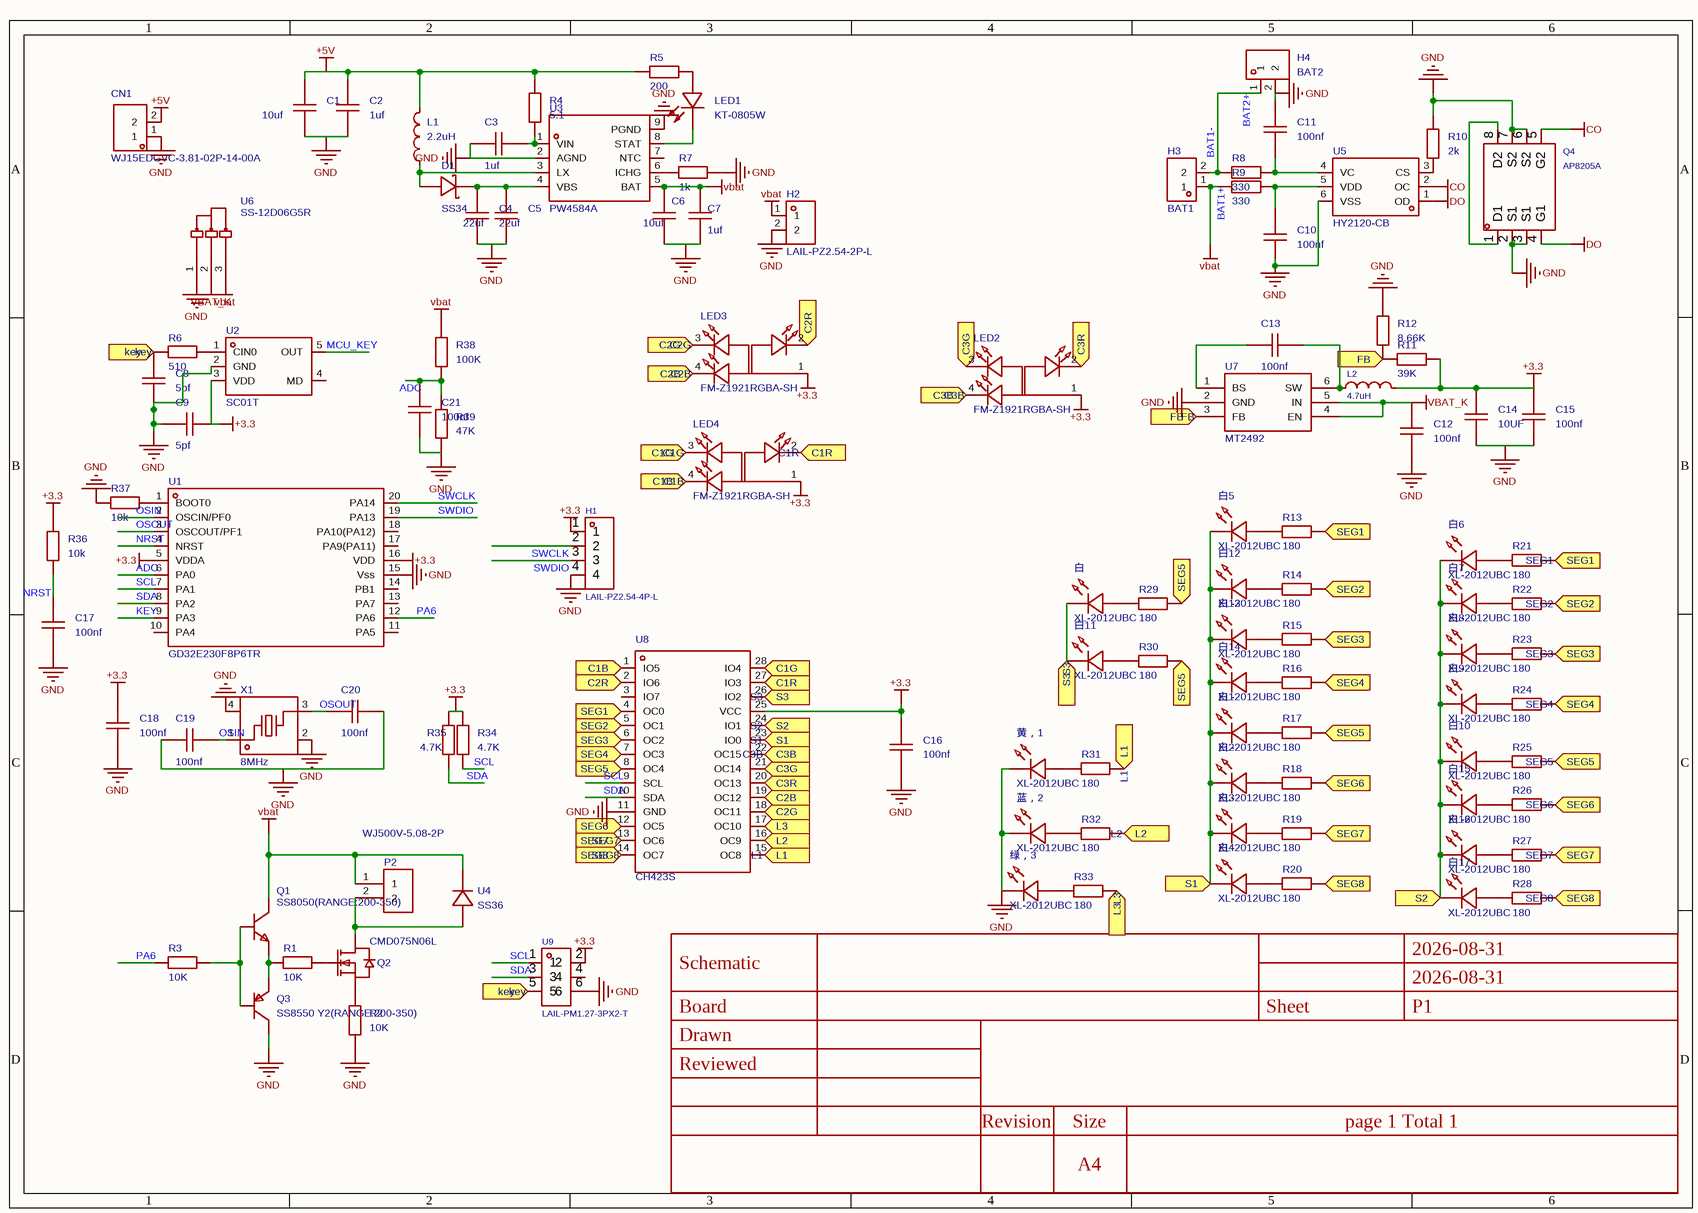
[diagram p0: MISC80546-2.schdoc]
# Altium schematic sheet MISC80546-2.schdoc
size 297 x 209 mm; Version: V1.0; @Project Name: MISC80546; @Update Date: 2026-08-31; @Create Date: 2026-08-31; @Board Name: MISC80546; @Create Time: 14:55:22; @Page Count: 1; @Page No: 1; @Schematic Name: MISC80546; @Update Time: 14:55:22; Size: A4

## Parts
C1  10uf  [C0603]
C2  1uf  [C0603]
C3  1uf  [C0603]
C4  22uf  [C0603]
C5  22uf  [C0603]
C6  10uf  [C0603]
C7  1uf  [C0603]
C8  5pf  [C0603]
C9  5pf  [C0603]
C10  100nf  [C0603]
C11  100nf  [C0603]
C12  100nf  [C0603]
C13  100nf  [C0603]
C14  10UF  [C0603]
C15  100nf  [C0603]
C16  100nf  [C0603]
C17  100nf  [C0603]
C18  100nf  [C0603]
C19  100nf  [C0603]
C20  100nf  [C0603]
C21  100nf  [C0603]
CN1  WJ15EDGVC-3.81-02P-14-00A  [CONN-TH_WJ15EDGVC-3.81-2P]
D1  SS34  [SMA_L4.3-W2.6-LS5.2-RD]
H1  LAIL-PZ2.54-4P-L  [CONN-TH_LAIL-PZ2.54-4P-L]
H2  LAIL-PZ2.54-2P-L  [CONN-TH_LAIL-PZ2.54-2P-L]
H3  BAT1  [CONN-TH_LAIL-PZ2.54-2P-L]
H4  BAT2  [CONN-TH_LAIL-PZ2.54-2P-L]
L1  2.2uH  [IND-SMD_L4.0-W4.0_LQH44PN2R2MP0L]
L2  4.7uH  [IND-SMD_L4.0-W4.0_SMNR4012]
LED1  KT-0805W  [LED0805-R-RD]
LED2  FM-Z1921RGBA-SH  [LED-ARRAY-SMD_4P-L2.2-W2.1-BR]
LED3  FM-Z1921RGBA-SH  [LED-ARRAY-SMD_4P-L2.2-W2.1-BR]
LED4  FM-Z1921RGBA-SH  [LED-ARRAY-SMD_4P-L2.2-W2.1-BR]
P2  WJ500V-5.08-2P  [CONN-TH_2P-P5.00_WJ500V-5.08-2P]
Q1  SS8050(RANGE:200-350)  [SOT-23-3_L2.9-W1.3-P1.90-LS2.4-BR]
Q2  CMD075N06L  [TO-252-2_L6.6-W6.1-P4.57-LS9.9-BR-CW]
Q3  SS8550 Y2(RANGE:200-350)  [SOT-23-3_L2.9-W1.3-P1.90-LS2.4-BR]
Q4  AP8205A  [TSSOP-8_L4.4-W3.0-P0.65-LS6.4-BL-2]
R1  10K  [R0603]
R2  10K  [R0603]
R3  10K  [R0603]
R4  5.1  [R0603]
R5  200  [R0603]
R6  510  [R0603]
R7  1k  [R0603]
R8  330  [R0603]
R9  330  [R0603]
R10  2k  [R0603]
R11  39K  [R0603]
R12  8.66K  [R0603]
R13  180  [R0603]
R14  180  [R0603]
R15  180  [R0603]
R16  180  [R0603]
R17  180  [R0603]
R18  180  [R0603]
R19  180  [R0603]
R20  180  [R0603]
R21  180  [R0603]
R22  180  [R0603]
R23  180  [R0603]
R24  180  [R0603]
R25  180  [R0603]
R26  180  [R0603]
R27  180  [R0603]
R28  180  [R0603]
R29  180  [R0603]
R30  180  [R0603]
R31  180  [R0603]
R32  180  [R0603]
R33  180  [R0603]
R34  4.7K  [R0603]
R35  4.7K  [R0603]
R36  10k  [R0603]
R37  10k  [R0603]
R38  100K  [R0603]
R39  47K  [R0603]
U1  GD32E230F8P6TR  [TSSOP-20_L6.5-W4.4-P0.65-LS6.4-BL]
U2  SC01T  [SOT-23-5_L2.9-W1.6-P0.95-LS2.8-BR]
U3  PW4584A  [ESOP-8_L4.9-W3.9-P1.27-LS6.0-BL-EP-1]
U4  SS36  [SMA_L4.3-W2.6-LS5.1-RD]
U5  HY2120-CB  [SOT-23-6_L2.9-W1.6-P0.95-LS2.8-BR]
U6  SS-12D06G5R  [SW-TH_SS-12D06G5R]
U7  MT2492  [SOT-23-6_L2.9-W1.6-P0.95-LS2.8-BL_3]
U8  CH423S  [SOP-28_L17.9-W7.5-P1.27-LS10.3-BL]
U9  LAIL-PM1.27-3PX2-T  [HDR-SMD_6P-P1.27_LAIL-PM1.27-3PX2-T]
X1  8MHz  [CRYSTAL-SMD_4P-L3.2-W2.5-BL]
白  XL-2012UBC  [LED0805-RD]
白1  XL-2012UBC  [LED0805-RD]
白2  XL-2012UBC  [LED0805-RD]
白3  XL-2012UBC  [LED0805-RD]
白4  XL-2012UBC  [LED0805-RD]
白5  XL-2012UBC  [LED0805-RD]
白6  XL-2012UBC  [LED0805-RD]
白7  XL-2012UBC  [LED0805-RD]
白8  XL-2012UBC  [LED0805-RD]
白9  XL-2012UBC  [LED0805-RD]
白10  XL-2012UBC  [LED0805-RD]
白11  XL-2012UBC  [LED0805-RD]
白12  XL-2012UBC  [LED0805-RD]
白13  XL-2012UBC  [LED0805-RD]
白14  XL-2012UBC  [LED0805-RD]
白15  XL-2012UBC  [LED0805-RD]
白16  XL-2012UBC  [LED0805-RD]
白17  XL-2012UBC  [LED0805-RD]
绿，3  XL-2012UBC  [LED0805-RD]
蓝，2  XL-2012UBC  [LED0805-RD]
黄，1  XL-2012UBC  [LED0805-RD]

## Ports
C1B (in), C1G (in), C1R (in), C2B (in), C2G (in), C2R (in), C3B (in), C3G (in), C3R (in), FB (in), key (in), L1 (in), L2 (in), L3 (in), S1 (in), S2 (in), S3 (in), SEG1 (in), SEG2 (in), SEG3 (in), SEG4 (in), SEG5 (in), SEG6 (in), SEG7 (in), SEG8 (in)

## Nets
+3.3: C9.1 C14.2 C15.2 C16.2 C18.1 H1.1 L2.2 LED2.1(+) LED3.1(+) LED4.1(+) R11.1 R34.2 R35.2 R36.2 U1.5(VDDA) U1.16(VDD) U2.3(VDD) U8.25(VCC) U9.2
+5V: C1.2 C2.2 CN1.2 L1.2 R4.2 R5.2
BAT1+: C6.1 C7.1 H2.1 H3.1 P2.1 Q1.3(C) R9.1 R38.2 U3.5(BAT) U4.1(K) U6.3  [also labelled vbat]
CO: Q4.5(G2) U5.2(OC)
DO: Q4.4(G1) U5.1(OD)
GND: C1.1 C2.1 C3.1 C4.2 C5.1 C6.2 C7.2 C8.1 C9.2 C10.1 C11.2 C12.1 C14.1 C15.1 C16.1 C17.2 C18.2 C19.2 C20.2 C21.2 CN1.1 H1.4 H2.2 H4.2 Q3.3(C) Q4.2(S1) Q4.3(S1) Q4.6(S2) Q4.7(S2) R2.1 R7.2 R10.2 R12.2 R37.2 R39.1 U1.15(Vss) U2.2(GND) U3.2(AGND) U3.9(PGND) U5.6(VSS) U6.1 U7.2(GND) U8.11(GND) U9.6 X1.2(GND) X1.4(GND) 绿，3.1(K) 蓝，2.1(K) 黄，1.1(K)
VBAT_K: C12.2 U6.2 U7.4(EN) U7.5(IN)
ADC: C21.1 R38.1 R39.2 U1.6(PA0)
BAT1-: H3.2 H4.1 R8.1  [also labelled BAT2+]
C1B: LED4.4(-) U8.1(IO5) ; port C1B
C1G: LED4.3(-) U8.28(IO4) ; port C1G
C1R: LED4.2(-) U8.27(IO3) ; port C1R
C2B: LED3.4(-) U8.19(OC12) ; port C2B
C2G: LED3.3(-) U8.18(OC11) ; port C2G
C2R: LED3.2(-) U8.2(IO6) ; port C2R
C3B: LED2.4(-) U8.22(OC15) ; port C3B
C3G: LED2.3(-) U8.21(OC14) ; port C3G
C3R: LED2.2(-) U8.20(OC13) ; port C3R
FB: R11.2 R12.1 U7.3(FB) ; port FB
KEY: C8.2 R6.1 U1.9(PA3) U9.5 ; port key
L1: R31.1 U8.15(OC8) ; port L1
L2: R32.1 U8.16(OC9) ; port L2
L3: R33.1 U8.17(OC10) ; port L3
MCU_KEY: U2.5(OUT)
NRST: C17.1 R36.1 U1.4(NRST)
OSIN: C19.1 U1.2(OSCIN/PF0) X1.1
OSOUT: C20.1 U1.3(OSCOUT/PF1) X1.3
PA6: R3.1 U1.12(PA6)
S1: U8.23(IO0) 白1.1(K) 白2.1(K) 白3.1(K) 白4.1(K) 白5.1(K) 白12.1(K) 白13.1(K) 白14.1(K) ; port S1
S2: U8.24(IO1) 白6.1(K) 白7.1(K) 白8.1(K) 白9.1(K) 白10.1(K) 白15.1(K) 白16.1(K) 白17.1(K) ; port S2
S3: U8.26(IO2) 白.1(K) 白11.1(K) ; port S3
SCL: R34.1 U1.7(PA1) U8.9(SCL) U9.1
SDA: R35.1 U1.8(PA2) U8.10(SDA) U9.3
SEG1: R13.1 R21.1 U8.4(OC0) ; port SEG1
SEG2: R14.1 R22.1 U8.5(OC1) ; port SEG2
SEG3: R15.1 R23.1 U8.6(OC2) ; port SEG3
SEG4: R16.1 R24.1 U8.7(OC3) ; port SEG4
SEG5: R17.1 R25.1 R29.1 R30.1 U8.8(OC4) ; port SEG5
SEG6: R18.1 R26.1 U8.12(OC5) ; port SEG6
SEG7: R19.1 R27.1 U8.13(OC6) ; port SEG7
SEG8: R20.1 R28.1 U8.14(OC7) ; port SEG8
SWCLK: H1.2 U1.20(PA14)
SWDIO: H1.3 U1.19(PA13)
NetC3_2: C3.2 R4.1 U3.1(VIN)
NetC4_1: C4.1 C5.2 D1.1(K) U3.4(VBS)
NetC10_2: C10.2 R9.2 U5.5(VDD)
NetC11_1: C11.1 R8.2 U5.4(VC)
NetC13_1: C13.1 L2.1 U7.6(SW)
NetC13_2: C13.2 U7.1(BS)
NetD1_2: D1.2(A) L1.1 U3.3(LX)
NetLED1_1: LED1.1(A) R5.1
NetLED1_2: LED1.2(K) U3.8(STAT)
NetP2_2: P2.2 Q2.2(D) U4.2(A)
NetQ1_1: Q1.1(B) Q3.1(B) R3.2
NetQ1_2: Q1.2(E) Q3.2(E) R1.1
NetQ2_1: Q2.1(G) R1.2
NetQ2_3: Q2.3(S) R2.2
NetQ4_1: Q4.1(D1) Q4.8(D2)
NetR6_2: R6.2 U2.1(CIN0)
NetR7_1: R7.1 U3.6(ICHG)
NetR10_1: R10.1 U5.3(CS)
NetR13_2: R13.2 白5.2(A)
NetR14_2: R14.2 白12.2(A)
NetR15_2: R15.2 白13.2(A)
NetR16_2: R16.2 白14.2(A)
NetR17_2: R17.2 白1.2(A)
NetR18_2: R18.2 白2.2(A)
NetR19_2: R19.2 白3.2(A)
NetR20_2: R20.2 白4.2(A)
NetR21_2: R21.2 白6.2(A)
NetR22_2: R22.2 白7.2(A)
NetR23_2: R23.2 白8.2(A)
NetR24_2: R24.2 白9.2(A)
NetR25_2: R25.2 白10.2(A)
NetR26_2: R26.2 白15.2(A)
NetR27_2: R27.2 白16.2(A)
NetR28_2: R28.2 白17.2(A)
NetR29_2: R29.2 白.2(A)
NetR30_2: R30.2 白11.2(A)
NetR31_2: R31.2 黄，1.2(A)
NetR32_2: R32.2 蓝，2.2(A)
NetR33_2: R33.2 绿，3.2(A)
NetR37_1: R37.1 U1.1(BOOT0)

Not connected (* = marked no-connect by the designer): U1 10(PA4) 11(PA5) 13(PA7) 14(PB1) 17(PA9(PA11)) 18(PA10(PA12)); U2 4(MD); U3 7(NTC); U8 3(IO7); U9 4

## Notes on the sheet
- 2026-08-31
- Schematic
- Board
- Sheet
- P1
- Drawn
- Reviewed
- Revision
- Size
- A4
- page 1 Total 1

## Library data of the parts
C1-C9 = CAP_0603: Symbol: Capacitance; ConvertToPcb: yes; ModelId: ac125912035d415993ca9572d50418b10819f05c4eef4c71ace90d822a990e87; ModelName: C0603_L1.6-W0.8-H0.8; ModelTransform: 62.992,31.496,0,0,0,0,0,0,0; Device: CAP_0603; AddInBom: yes; Supplier Footprint: 0603; FootprintName: C0603
  C1 C6: Value: 10uf
  C2 C3 C7: Value: 1uf
  C4 C5: Value: 22uf
  C8 C9: Value: 5pf
C10-C21 = CAP_0603: Symbol: Capacitance; 3D Model: ac125912035d415993ca9572d50418b10819f05c4eef4c71ace90d822a990e87; 3D Model Transform: 62.992,31.496,0,0,0,0,0,0,0; ConvertToPcb: yes; ModelName: C0603_L1.6-W0.8-H0.8; Device: CAP_0603; Supplier Footprint: 0603; AddInBom: yes; FootprintName: C0603
  C10-C13 C15-C21: Value: 100nf
  C14: Value: 10UF
CN1 = WJ15EDGVC-3.81-02P-14-00A: 连接器类型:板端/插座-闭口;固定方式:无固定装置;结构:1x2P;间距:3.81mm;颜色:绿色;安装方式:直插;排数:1;每排PIN数:2;额定电流:8A;额定电压:300V;线规 - AWG:-;线规 - 平方毫米:-;工作温度:-40℃~+105℃;; Manufacturer: KANGNEX(康奈克斯电气); Symbol: WJ15EDGVC-3.81-2P; AddInBom: yes; ModelId: 4fb8508385d5450abf2abd114199f87c0819f05c4eef4c71ace90d822a990e87; ModelName: CONN-TH_DB3.81-LI-2P; ModelTransform: 334.645,275.629,0,180,0,0,0,-27.559,-145.669; Connector Type: Board end/socket - closed; Number of Positions or Pins: 1x2P; Pitch: 3.81mm; Number of PINs Per Row: 2; Current Rating: 8A; Voltage Rating (Max): 300V; Device: WJ15EDGVC-3.81-02P-14-00A; LCSC Part Name: 无固定装置 1x2P 3.81mm 排数:1 每排P数:2; SupplierPart: C8396; ManufacturerPart: WJ15EDGVC-3.81-02P-14-00A; Supplier Footprint: 插件,P=3.81mm; JLCPCB Part Class: Extended Part; Datasheet: example.com/datasheet/WJ15EDGVC-3.81-02P-14-00A/8890.html; Supplier: LCSC; ConvertToPcb: yes; FootprintName: CONN-TH_WJ15EDGVC-3.81-2P; Termination Style: No fixing device; Color: Green; Mounting Type: Through-hole; Number of Pins: 2P; Number of Rows: 1; Wire Gauge - AWG: -; Wire Gauge - mm2: -; Operating Temperature: -40℃~+105℃; Connection Type: -; Outlet Direction (Vertical Basis): -
D1 = SS34_C8678: Diode configuration: single; forward voltage (Vf): 550mV@3A; DC reverse voltage (Vr): 40V; rectified current: 3A;; Manufacturer: MDD(辰达半导体); AddInBom: yes; ModelId: e3551acb3c5a4975a5e9d36087fe1fa20819f05c4eef4c71ace90d822a990e87; ModelTransform: 185.039,102.362,0,0,0,0,0,0,0; Reverse Leakage Current (Ir): 500uA@40V; Operating Junction Temperature Range: -55℃~+125℃; Symbol: SS34_C8678; Device: SS34_C8678; LCSC Part Name: 电压:40V 电流:3A; SupplierPart: C8678; ManufacturerPart: SS34; Supplier Footprint: SMA(DO-214AC); JLCPCB Part Class: Basic Part; Datasheet: example.com/datasheet/SS34/9178.html; Supplier: LCSC; ConvertToPcb: yes; FootprintName: SMA_L4.3-W2.6-LS5.2-RD; ModelName: SMA_L4.3-W2.6-LS5.2-RD; Diode Configuration: Single; Voltage - Forward(Vf@If): 550mV@3A; Voltage - DC Reverse(Vr): 40V; Current - Rectified: 3A
H1 = LAIL-PZ2.54-4P-L: Pin structure: 1x4P; pitch: 2.54mm; round/square pin: square pin; rows: single row; total pin positions: 4P; rated current: 3A; rated voltage: 250V; plastic height: 2.5mm; tail length: 3mm; contact material: brass; contact plating: gold; operating temperature: -25℃~+80℃; color: black;; Manufacturer: 莱联; AddInBom: yes; ModelId: 112b012cb4004446aa5386c9c86d05f00819f05c4eef4c71ace90d822a990e87; ModelTransform: 400.039,100,0,0,0,0,0,0,-118.11; Symbol: LAIL-PZ2.54-4P-L; Device: LAIL-PZ2.54-4P-L; LCSC Part Name: 1x4P 间距:2.54mm 方针; SupplierPart: C54950602; ManufacturerPart: LAIL-PZ2.54-4P-L; Supplier Footprint: 插件,P=2.54mm; JLCPCB Part Class: Extended Part; Datasheet: example.com/datasheet/LAIL-PZ2.54-4P-L/58519955.html; Supplier: LCSC; ConvertToPcb: yes; FootprintName: CONN-TH_LAIL-PZ2.54-4P-L; ModelName: CONN-TH_LAIL-PZ2.54-4P-L; Pin Structure: 1x4P; Pitch: 2.54mm; Circluar Pins/Square Pins: Square pin; Number of Rows: Single row; Number of Pins: 4P; Current Rating: 3A; Voltage Rating (Max): 250V; Insulation Height: 2.5mm; Length of End Connection Pin: 3mm; Contact Material: Brass; Contact Plating: Gold; Operating Temperature: -25℃~+80℃; Color: Black
H2-H4 = LAIL-PZ2.54-2P-L: Pin structure: 1x2P; pitch: 2.54mm; round/square pin: square pin; rows: single row; total pin positions: 2P; rated current: 3A; rated voltage: 250V; plastic height: 2.5mm; tail length: 3mm; contact material: brass; contact plating: gold; operating temperature: -25℃~+80℃; color: black;; Manufacturer: 莱联; AddInBom: yes; Symbol: LAIL-PZ2.54-2P-L; Device: LAIL-PZ2.54-2P-L; LCSC Part Name: 1x2P 间距:2.54mm 方针; Supplier Footprint: 插件,P=2.54mm; JLCPCB Part Class: Extended Part; Datasheet: example.com/datasheet/LAIL-PZ2.54-2P-L/58519956.html; Supplier: LCSC; Pin Structure: 1x2P; Pitch: 2.54mm; Circluar Pins/Square Pins: Square pin; Number of Rows: Single row; Number of Pins: 2P; Current Rating: 3A; Voltage Rating (Max): 250V; Insulation Height: 2.5mm; Length of End Connection Pin: 3mm; Contact Material: Brass; Contact Plating: Gold; Operating Temperature: -25℃~+80℃; Color: Black; ConvertToPcb: yes; FootprintName: CONN-TH_LAIL-PZ2.54-2P-L
  H2: Supplier Part: C54950603; Manufacturer Part: LAIL-PZ2.54-2P-L
  H3: Manufacturer Part: BAT1; SupplierPart: C54950603
  H4: Manufacturer Part: BAT2; SupplierPart: C54950603
L1 = SMNR4020-2.2UH: Inductance: 2.2uH; tolerance: ±20%; rated current: 3.4A; saturation current (Isat): 3.4A;; Manufacturer: SXN(顺翔诺); AddInBom: yes; ModelId: 0a0a6aed311d407c9209933687c5f1ec0819f05c4eef4c71ace90d822a990e87; ModelName: IND-SMD_L4.0-W4.0-H1.65; ModelTransform: 157.48,157.484,0,0,0,0,0,0,0; DC Resistance(DCR): 46mΩ; Symbol: SMNR4020-2.2UH; Device: SMNR4020-2.2UH; LCSC Part Name: 2.2uH ±20% 3.4A; SupplierPart: C135262; ManufacturerPart: SMNR4020-2.2UH; Supplier Footprint: SMD,4x4mm; JLCPCB Part Class: Extended Part; Datasheet: example.com/datasheet/SMNR4020-2.2UH/146573.html; Supplier: LCSC; ConvertToPcb: yes; FootprintName: IND-SMD_L4.0-W4.0_LQH44PN2R2MP0L; Value: 2.2uH; Tolerance: ±20%; Current Rating: 3.4A; Current - Saturation(Isat): 3.4A
L2 = PNR4030-4R7-M: Inductance: 4.7uH; tolerance: ±20%; rated current: 2.3A; saturation current (Isat): 3.2A; type: magnetic-glue shielded inductor;; Manufacturer: JIERR(捷而瑞); AddInBom: yes; ModelId: a0312046766d423b9f3ce3b362dc752d0819f05c4eef4c71ace90d822a990e87; ModelName: IND-SMD_L4.0-W4.0-H3.0; ModelTransform: 157.48,158.267,0,90,0,0,0,0,0; DC Resistance(DCR): 60mΩ; Symbol: PNR4030-4R7-M; Device: PNR4030-4R7-M; LCSC Part Name: 4.7uH±20% 3.2A; SupplierPart: C55381754; ManufacturerPart: PNR4030-4R7-M; Supplier Footprint: SMD,4x4mm; JLCPCB Part Class: Extended Part; Datasheet: example.com/datasheet/PNR4030-4R7-M/59339382.html; Supplier: LCSC; ConvertToPcb: yes; FootprintName: IND-SMD_L4.0-W4.0_SMNR4012; Value: 4.7uH; Tolerance: ±20%; Current Rating: 2.3A; Current - Saturation(Isat): 3.2A; Type: Magnetic-glue shielded inductor
LED1 = KT-0805W: Lamp holder type: 2mmx1.25mm square holder; illumination color: white; forward voltage (Vf): 2.6V~3.2V; power: 80mW; forward current: 25mA; wavelength: -; diode configuration: single diode; lens color: yellow lens; color temperature: 13172K~100000K; luminous intensity: 350mcd; viewing angle: 120°; carrier tape: top mount; operating temperature: -30℃~+85℃;; Manufacturer: KENTO; Symbol: whiteLEDSMD; AddInBom: yes; ModelId: 6ccd75a2b5134d6ab756ecf3c14a72900819f05c4eef4c71ace90d822a990e87; ModelName: LED0805-RD; ModelTransform: 79.527,49.2125,0,0,0,0,0,0,0; Device: KT-0805W; LCSC Part Name: 0805 白灯 高亮; SupplierPart: C34499; ManufacturerPart: KT-0805W; Supplier Footprint: 0805; JLCPCB Part Class: Basic Part; Datasheet: example.com/datasheet/KT-0805W/35468.html; Supplier: LCSC; ConvertToPcb: yes; FootprintName: LED0805-R-RD; Lamp Holder Type: 2mmx1.25mm square holder; Illumination Color: White; Voltage - Forward(Vf): 2.6V~3.2V; Power(Watts): 80mW; Forward Current: 25mA; Wavelength - Dominant: -; Peak Wavelength: -; Diode Configuration: Single diode; Lens Color: Yellow lens; Color Temperature: 13172K~100000K; Luminous Intensity: 350mcd; Viewing Angle: 120°; Mounting Style: Top-mount; Operating Temperature: -30℃~+85℃
LED2-LED4 = FM-Z1921RGBA-SH: Outdoor gold-wire RGB, black outside white inside design, high contrast; Manufacturer: 国星光电; AddInBom: yes; ModelId: 94ecc57fe6f245a7af3ffe8c67617d540819f05c4eef4c71ace90d822a990e87; ModelTransform: 84.6455,80.709,0,0,0,0,0,0.005,0; Diode Configuration: Common anode; Dominant Wavelength - R: 615nm~630nm; Dominant Wavelength - G: 515nm~535nm; Dominant Wavelength - B: 465nm~480nm; Viewing Angle: 110°; Installation Method: Top-mount; Luminous Intensity - R: 300mcd~680mcd; Luminous Intensity - G: 480mcd~1100mcd; Luminous Intensity - B: 70mcd~160mcd; Forward Voltage(Vf) - R: 1.8V~2.4V; Forward Voltage(Vf) - G: 2.4V~3.4V; Forward Current - R: 15mA; Forward Current - G: 8mA; Forward Current - B: 5mA; Power(Watts) - R: 60mW; Power(Watts) - G: 85mW; Symbol: FM-Z1921RGBA-SH; Device: FM-Z1921RGBA-SH; LCSC Part Name: TOP全彩LED; SupplierPart: C2874120; ManufacturerPart: FM-Z1921RGBA-SH; Supplier Footprint: SMD-4P,2.2x2.1mm; JLCPCB Part Class: Extended Part; Datasheet: example.com/datasheet/FM-Z1921RGBA-SH/3078832.html; Supplier: LCSC; ConvertToPcb: yes; FootprintName: LED-ARRAY-SMD_4P-L2.2-W2.1-BR; ModelName: LED-ARRAY-SMD_4P-L2.2-W2.1-BR; Lens Color: -; Antistatic Capacity: -; Peak Wavelength - R: -; Peak Wavelength - G: -; Peak Wavelength - B: -; Operating Temperature: -30℃~+85℃; Lamp Holder Type: -; Length: 2.15mm; Width: 2.05mm; Height: 1.9mm; Pitch: -; Forward Voltage(Vf) - B: 2.4V~3.4V; Power(Watts) - B: 85mW
P2 = WJ500V-5.08-2P: 结构:1x2P;间距:5.08mm;颜色:绿色;安装类型:直插;排数:1;每排PIN数:2;额定电流:18A;额定电压:250V;线规 - AWG:14~30;线规 - 平方毫米:2.5;工作温度:-40℃~+105℃;; Manufacturer: KANGNEX(康奈克斯电气); Symbol: WJ500V-5.08-2P-14-00A; 3D Model: 0f4a503c8d3b4ae19ed61267f5e9a1d70819f05c4eef4c71ace90d822a990e87; 3D Model Transform: 423.621,393.7,0,0,0,0,-11.811,19.685,-137.795; Number of Positions or Pins: 1x2P; Pitch: 5.08mm; Number of PINs Per Row: 2; Screw Specification: M2.5; Current Rating: 18A; Voltage Rating (Max): 250V; Wire Gauge - AWG: 14~30; Wire Gauge - mm2: 2.5; AddInBom: yes; Device: WJ500V-5.08-2P; LCSC Part Name: 1x2P 5.08mm 直插 排数:1 每排P数:2; Supplier Part: C8465; Manufacturer Part: WJ500V-5.08-2P; Supplier Footprint: 插件,P=5.08mm; JLCPCB Part Class: Extended Part; Datasheet: example.com/datasheet/WJ500V-5.08-2P/8959.html; Supplier: LCSC; Color: Green; Mounting Type: Through-hole; Number of Pins: 2P; Number of Rows: 1; Operating Temperature: -40℃~+105℃; ConvertToPcb: yes; FootprintName: CONN-TH_2P-P5.00_WJ500V-5.08-2P; ModelName: CONN-TH_2P-P5.00_WJ500V-5.08-2P
Q1 = SS8050(RANGE:200-350)_C2150: Transistor type: NPN; collector current (Ic): 1.5A; collector-emitter breakdown voltage (Vceo): 25V; power dissipation (Pd): 300mW; DC current gain (hFE): 200@800mA,1V;; Manufacturer: CJ(江苏长电/长晶); Symbol: SS8050_C2150; 3D Model: c62791f0466c4ae2a892c056b845b0ca0819f05c4eef4c71ace90d822a990e87; 3D Model Transform: 98.425,114.173,0,180,0,0,0.0005,-0.0005,0; Transition frequency(fT): 100MHz; Current - Collector Cutoff: 100nA; Vce Saturation(VCE(sat)): 500mV@800mA,80mA; Emitter-Base Voltage(Vebo): 5V; Number: 1 NPN; AddInBom: yes; ModelName: SOT-23-3P_L2.9-W1.3-H1.0-LS2.4-P0.95; Device: SS8050(RANGE:200-350)_C2150; LCSC Part Name: hfe=200~350 NPN 电流:1.5A 电压:25V; Supplier Part: C2150; Manufacturer Part: SS8050(RANGE:200-350); Supplier Footprint: SOT-23; JLCPCB Part Class: Basic Part; Datasheet: example.com/datasheet/SS8050(RANGE%253A200-350)/2507.html; Supplier: LCSC; type: NPN; Current - Collector(Ic): 1.5A; Collector - Emitter Voltage VCEO: 25V; Pd - Power Dissipation: 300mW; DC Current Gain: 200@800mA,1V; Operating Temperature: -55℃~+150℃; ConvertToPcb: yes; FootprintName: SOT-23-3_L2.9-W1.3-P1.90-LS2.4-BR
Q2 = CMD075N06L: MOS管,封装：TO-252，电压：60V,电流：90A,10V内阻：0.0075欧，4.5V内阻：0.011欧，功率：130W，Cisstyp:2100pF; Manufacturer: Cmos(广东场效应半导体); 3D Model: ce57f84d66384067af8a68020b6de06d0819f05c4eef4c71ace90d822a990e87; 3D Model Transform: 259.842,390.52442,0,90,0,0,-39.39,0,0; AddInBom: yes; ModelName: TO-252-2L-3P_L6.6-W6.1-H2.3-LS10.1-P4.6; Symbol: CMD075N06L; Device: CMD075N06L; LCSC Part Name: MOS管 TO-252 60V 90A; Supplier Part: C54951111; Manufacturer Part: CMD075N06L; Supplier Footprint: TO-252; JLCPCB Part Class: Extended Part; Datasheet: example.com/datasheet/CMD075N06L/58522671.html; Supplier: LCSC; ConvertToPcb: yes; FootprintName: TO-252-2_L6.6-W6.1-P4.57-LS9.9-BR-CW
Q3 = SS8550 Y2(RANGE:200-350): Transistor type: PNP; collector current (Ic): 1.5A; collector-emitter breakdown voltage (Vceo): 25V; power (Pd): 300mW; DC current gain (hFE@Ic,Vce): 200@100mA,1V;; Manufacturer: CJ(江苏长电/长晶); Symbol: SS8550_C8542; 3D Model: c62791f0466c4ae2a892c056b845b0ca0819f05c4eef4c71ace90d822a990e87; 3D Model Transform: 98.425,114.173,0,180,0,0,0.0005,-0.0005,0; Transition Frequency (fT): 100MHz; Collector Cut-Off Current (Icbo): 100nA; Collector-Emitter Saturation Voltage (VCE(sat)@Ic,Ib): 500mV@800mA,80mA; AddInBom: yes; ModelName: SOT-23-3P_L2.9-W1.3-H1.0-LS2.4-P0.95; Device: SS8550 Y2(RANGE:200-350); LCSC Part Name: PNP 电流:1.5A 耐压:25V hfe=200~350; Supplier Part: C8542; Manufacturer Part: SS8550 Y2(RANGE:200-350); Supplier Footprint: SOT-23; JLCPCB Part Class: Basic Part; Datasheet: example.com/upload/public/pdf/source/20140809/1457707214734.pdf; Supplier: LCSC; Transistor Type: PNP; Collector Current (Ic): 1.5A; Collector-Emitter Breakdown Voltage (Vceo): 25V; Power Dissipation (Pd): 300mW; DC Current Gain (hFE@Ic,Vce): 200@100mA,1V; Operating Temperature: -55℃~+150℃; ConvertToPcb: yes; FootprintName: SOT-23-3_L2.9-W1.3-P1.90-LS2.4-BR
Q4 = AP8205A: Quantity: 2 N-channel; drain-source voltage (Vdss): 20V; continuous drain current (Id): 6A; on-resistance (RDS(on)): 36mΩ@2.5V; power dissipation (Pd): 1.5W; threshold voltage (Vgs(th)): 1.2V;; Manufacturer: ALLPOWER(铨力); AddInBom: yes; ModelId: 2d0fd2703afb4f81a9dfc54e2181a6240819f05c4eef4c71ace90d822a990e87; ModelTransform: 118.11,251.968,0,0,0,0,0,0,0; Input Capacitance(Ciss): 1.035nF; Reverse Transfer Capacitance (Crss@Vds): 150pF; Output Capacitance(Coss): 320pF; Symbol: AP8205A; Device: AP8205A; LCSC Part Name: 2个N沟道 耐压:20V 电流:6A; SupplierPart: C360341; ManufacturerPart: AP8205A; Supplier Footprint: TSSOP-8; JLCPCB Part Class: Extended Part; Datasheet: example.com/datasheet/AP8205A/335328.html; Supplier: LCSC; ConvertToPcb: yes; FootprintName: TSSOP-8_L4.4-W3.0-P0.65-LS6.4-BL-2; ModelName: TSSOP-8_L4.4-W3.0-P0.65-LS6.4-BL-2; Number: 2 N-channel; Drain to Source Voltage: 20V; Current - Continuous Drain(Id): 6A; RDS(on): 36mΩ@2.5V; Pd - Power Dissipation: 1.5W; Gate Threshold Voltage (Vgs(th)): 1.2V; Operating Temperature: -55℃~+150℃; Configuration: -; Type: N-channel
R1-R39 = Res_0603: Symbol: Resistor; 3D Model: fc143cca1e79419f9cd78b61e9279f080819f05c4eef4c71ace90d822a990e87; 3D Model Transform: 31.8897,63.7794,0,90,0,0,0,0,0; ConvertToPcb: yes; Device: Res_0603; Supplier Footprint: 0603; AddInBom: yes; FootprintName: R0603; ModelName: R0603
  R1-R3: Value: 10K
  R4: Value: 5.1
  R5: Value: 200
  R6: Value: 510
  R7: Value: 1k
  R8 R9: Value: 330
  R10: Value: 2k
  R11: Value: 39K
  R12: Value: 8.66K
  R13-R33: Value: 180
  R34 R35: Value: 4.7K
  R36 R37: Value: 10k
  R38: Value: 100K
  R39: Value: 47K
U1 = GD32E230F8P6TR: CPU core: ARM Cortex-M series; max CPU frequency: 72MHz;; Manufacturer: GigaDevice(兆易创新); AddInBom: yes; ModelId: c491f68934b34c649df5890a1d97cd0f0819f05c4eef4c71ace90d822a990e87; ModelName: TSSOP-20_L6.5-W4.4-H1.0-LS6.4-P0.65; ModelTransform: 251.969,255.906,0,90,0,0,0.0005,0,0; Program Storage Size: 64KB; Program Memory Type: FLASH; Number of I/O: 15; ADC (Bit): 12bit; Voltage - Supply: 1.8V~3.6V; Symbol: GD32E230F8P6TR; Device: GD32E230F8P6TR; LCSC Part Name: ARM Cortex-M23 32位微控制器（MCU）; SupplierPart: C380785; ManufacturerPart: GD32E230F8P6TR; Supplier Footprint: TSSOP-20; JLCPCB Part Class: Extended Part; Datasheet: example.com/datasheet/GD32E230F8P6TR/352997.html; Supplier: LCSC; ConvertToPcb: yes; FootprintName: TSSOP-20_L6.5-W4.4-P0.65-LS6.4-BL; CPU Core: ARM Cortex-M series; CPU Maximum Speed: 72MHz
U2 = SC01T: Channels: 1; features: capacitive touch; automatic sensitivity calibration; self-locking: yes;; Manufacturer: icman(晶尊微); ModelId: 7ba65df16e7b4570af156e925f9c37fe0819f05c4eef4c71ace90d822a990e87; ModelTransform: 114.173,114.173,0,90,0,0,0,0,0; Number of Channels: 1; Voltage - Supply: 2V~6.5V; Current - Supply: 43uA; Standby Current: 4uA; Symbol: SC01T; Device: SC01T; LCSC Part Name: 单通道带自校正功能的容性触摸感应器; SupplierPart: C2930882; ManufacturerPart: SC01T; Supplier Footprint: SOT-23-5; JLCPCB Part Class: Extended Part; Datasheet: example.com/datasheet/SC01T/3268715.html; Supplier: LCSC; AddInBom: yes; ConvertToPcb: yes; FootprintName: SOT-23-5_L2.9-W1.6-P0.95-LS2.8-BR; ModelName: SOT-23-5_L2.9-W1.6-P0.95-LS2.8-BR; Features: Capacitive touch; automatic sensitivity calibration; Whether the Lock: Yes; Operating Temperature: -40℃~+85℃
U3 = PW4584A: AddInBom: yes; ModelId: 1edf17d9e1eb44b9aabe355eb95382d10819f05c4eef4c71ace90d822a990e87; ModelTransform: 192.913,236.22,0,0,0,0,0,0,0; Symbol: PW4584A; Device: PW4584A; LCSC Part Name: PW4584A; SupplierPart: C9900207824; ManufacturerPart: PW4584A; Supplier Footprint: SOP8-EP; Supplier: LCSC; ConvertToPcb: yes; FootprintName: ESOP-8_L4.9-W3.9-P1.27-LS6.0-BL-EP-1; ModelName: ESOP-8_L4.9-W3.9-P1.27-LS6.0-BL-EP-1
U4 = SS36: Symbol: SS36_C9900010124; 3D Model: 1d20a911e9694ba6aaf6e9207164e4da0819f05c4eef4c71ace90d822a990e87; 3D Model Transform: 196.4563,102.362,0,0,0,0,0.001,-0.001,0; AddInBom: yes; Device: SS36; LCSC Part Name: SS36; Supplier Part: C9900010124; Manufacturer Part: SS36; Supplier Footprint: SMA_L4.3-W2.6-LS5.1-RD; JLCPCB Part Class: Extended Part; Supplier: LCSC; ConvertToPcb: yes; FootprintName: SMA_L4.3-W2.6-LS5.1-RD; ModelName: SMA_L4.3-W2.6-LS5.1-RD
U5 = HY2120-CB: Operating voltage: 1.5V~10V; max charge current: -; battery type: lithium battery; battery cells: 2;; Manufacturer: HYCON(宏康); Symbol: HY2120CB; AddInBom: yes; ModelId: 18da8f6c14a34920b3e136b5c401a1190819f05c4eef4c71ace90d822a990e87; ModelName: SOT-23-6_L2.9-W1.6-H1.5-LS2.8-P0.95; ModelTransform: 110.73671,114.173,0,180,0,0,0.001,-0.003,0; The Chip Type: Protection IC; Charging Saturation Voltage: 4.28V; End-Off Voltage: 2.9V; Number of Cells: 2; Battery Temperature Detection: Not supported; 0V Battery Charge: Supported; Supply Current (Iq): 100nA; Device: HY2120-CB; LCSC Part Name: 2节锂离子/锂聚合物电池组保护IC; SupplierPart: C116509; ManufacturerPart: HY2120-CB; Supplier Footprint: SOT-23-6; JLCPCB Part Class: Extended Part; Datasheet: example.com/datasheet/HY2120-CB/117763.html; Supplier: LCSC; ConvertToPcb: yes; FootprintName: SOT-23-6_L2.9-W1.6-P0.95-LS2.8-BR; Voltage - Supply: 1.5V~10V; Charge Current - Max: -; Type of Battery: Lithium battery; Operating Temperature: -40℃~+85℃; Balance Current: -; Interface: -; Features: -
U6 = SS-12D06G5R: 电路结构:单刀双掷;安装方式:弯插;开关颜色:红色;额定电流:3A;额定电压:125V;工作寿命:1万次;; Manufacturer: XKB Connection(中国星坤); AddInBom: yes; ModelId: f91debf9c26a45d786769adcf7904fe10819f05c4eef4c71ace90d822a990e87; ModelTransform: 510.2352,633.85696,0,180,0,0,-0.002,-291.339,-98.425; Circuit: SPDT; Actuator Style: Rectangular post; Actuator Color: Red; Current Rating: 3A; Voltage Rating: 125V; Life: 1万次; Symbol: SS-12D06G5R; Device: SS-12D06G5R; LCSC Part Name: SS-12D06G5R; SupplierPart: C5146583; ManufacturerPart: SS-12D06G5R; Supplier Footprint: 弯插-3P,13x6.6mm; JLCPCB Part Class: Extended Part; Datasheet: example.com/datasheet/SS-12D06G5R/5769292.html; Supplier: LCSC; ConvertToPcb: yes; FootprintName: SW-TH_SS-12D06G5R; ModelName: SW-TH_SS-12D06G5R; Termination Style: PC pin; Length: 12.95mm; Width: 6.6mm; Mounting Type: Right-angle
U7 = MT2492: Function type: step-down; operating voltage: 4.5V~16V; output voltage: -; output current: 2A; output type: adjustable;; Manufacturer: 西安航天民芯; AddInBom: yes; ModelId: fb8f66c7218e47258c3712467298ba040819f05c4eef4c71ace90d822a990e87; ModelTransform: 114.173,110.236,0,0,0,0,0,0,0; Frequency - Switching: 600kHz; Number of Outputs: 1; Quiescent Current: 300uA; Switch tube (built-in/external): Built-in; Symbol: MT2492; Device: MT2492; LCSC Part Name: 降压型 2A 4.5V~16V; SupplierPart: C89358; ManufacturerPart: MT2492; Supplier Footprint: SOT-23-6; JLCPCB Part Class: Extended Part; Datasheet: example.com/datasheet/MT2492/90538.html; Supplier: LCSC; ConvertToPcb: yes; FootprintName: SOT-23-6_L2.9-W1.6-P0.95-LS2.8-BL_3; ModelName: SOT-23-6_L2.9-W1.6-P0.95-LS2.8-BL_3; Function: Step-down; Voltage - Supply: 4.5V~16V; Output Voltage: -; Output Current: 2A; Operating Temperature: -40℃~+85℃@(TA); Synchronous Rectifier: Yes; Topology: Step-down; Output Type: Adjustable; Features: Light-load high-efficiency mode; cycle-by-cycle current limit; overcurrent protection; hiccup current limit
U8 = CH423S: Interface type: -; I/O count: 8; clock frequency (fc): 1MHz;; Manufacturer: WCH(南京沁恒); AddInBom: yes; ModelId: 4632410aaaee431280089e18ae3ace4b0819f05c4eef4c71ace90d822a990e87; ModelTransform: 704.723,405.511,0,0,0,0,0,0,0; Number of I/O: 8; Voltage - Supply: 3V~5V; Symbol: CH423S; Device: CH423S; LCSC Part Name: 两线远程 I/O扩展芯片; SupplierPart: C111663; ManufacturerPart: CH423S; Supplier Footprint: SOP-28-300mil; JLCPCB Part Class: Extended Part; Datasheet: example.com/datasheet/CH423S/112891.html; Supplier: LCSC; ConvertToPcb: yes; FootprintName: SOP-28_L17.9-W7.5-P1.27-LS10.3-BL; ModelName: SOP-28_L17.9-W7.5-P1.27-LS10.3-BL; Interface: -; Interrupt Output: -; Output Type: -; Current - Output Low(IOL): -; Current - Output High(IOH): -; Clock Frequency: 1MHz; Operating Temperature: -40℃~+85℃
U9 = LAIL-PM1.27-3PX2-T: Socket structure: 2x3P; pitch: 1.27mm; row spacing: 1.27mm; round/square hole: square hole; rows: double row; total hole positions: 6P; rated current: 1A; rated voltage: 250V; socket direction: top; plastic height: 4.3mm; contact material: phosphor bronze; contact plating: gold; operating temperature: -25℃~+80℃;; Manufacturer: 莱联; AddInBom: yes; Symbol: LAIL-PM1.27-3PX2-T; Device: LAIL-PM1.27-3PX2-T; LCSC Part Name: 2x3P 间距:1.27mm; SupplierPart: C54973809; ManufacturerPart: LAIL-PM1.27-3PX2-T; Supplier Footprint: SMD,P=1.27mm; JLCPCB Part Class: Extended Part; Datasheet: example.com/datasheet/LAIL-PM1.27-3PX2-T/58554887.html; Supplier: LCSC; ConvertToPcb: yes; FootprintName: HDR-SMD_6P-P1.27_LAIL-PM1.27-3PX2-T; Holes Structure: 2x3P; Pitch: 1.27mm; Row Spacing: 1.27mm; Circular Hole / Square Hole: Square hole; Number of Rows: Double row; Number of Positions: 6P; Current Rating: 1A; Voltage Rating (Max): 250V; Holes Direction: Top; Insulation Height: 4.3mm; Contact Material: Phosphor bronze; Contact Plating: Gold; Operating Temperature: -25℃~+80℃
X1 = XL2EL89CSI-KPIYLC-8M: Crystal type: SMD crystal; frequency: 8MHz; frequency deviation at room temperature: ±10ppm; load capacitance: 20pF; frequency stability: ±20ppm;; Manufacturer: YXC(扬兴晶振); AddInBom: yes; ModelId: ff2dfd5650294453a14147960efe18380819f05c4eef4c71ace90d822a990e87; ModelTransform: 125.984,98.425,0,0,0,0,0,0,0; Equivalent Series Resistance(ESR): 180Ω; Symbol: XL2EL89CSI-KPIYLC-8M; Device: XL2EL89CSI-KPIYLC-8M; LCSC Part Name: YSX321SL 8MHZ 4P 3225 20PF ±10PPM -40~85℃ (±20PPM); SupplierPart: C42400161; ManufacturerPart: XL2EL89CSI-KPIYLC-8M; Supplier Footprint: SMD3225-4P; JLCPCB Part Class: Extended Part; Datasheet: example.com/datasheet/XL2EL89CSI-KPIYLC-8M/44352056.html; Supplier: LCSC; ConvertToPcb: yes; FootprintName: CRYSTAL-SMD_4P-L3.2-W2.5-BL; ModelName: CRYSTAL-SMD_4P-L3.2-W2.5-BL; Type: SMD crystal; Value: 8MHz; Normal temperature Frequency Tolerance: ±10ppm; Load Capacitance: 20pF; Frequency Stability: ±20ppm; Operating Temperature: -40℃~+85℃
白 白1-白17 = XL-2012UBC: Lamp holder type: 2.0mmx1.2mm square holder; illumination color: blue; forward voltage (Vf): 3.2V; power: 70mW; forward current: 20mA; wavelength: 460nm~475nm; diode configuration: single diode; lens color: colorless transparent lens; color temperature: -; luminous intensity: 260mcd; viewing angle: 120°; carrier tape: top mount; operating temperature: -40℃~+85℃;; Manufacturer: XINGLIGHT(成兴光); 3D Model: b1c5ed7a4f6e46d3bc6f6cc7c20f3fea0819f05c4eef4c71ace90d822a990e87; 3D Model Transform: 79.527,49.2125,0,0,0,0,0,0,0; Peak Wavelength: 470nm; AddInBom: yes; Symbol: XL-2012UBC; Device: XL-2012UBC; LCSC Part Name: 0805蓝贴片式发光二极管; Supplier Part: C965817; Manufacturer Part: XL-2012UBC; Supplier Footprint: 0805; JLCPCB Part Class: Extended Part; Datasheet: example.com/datasheet/XL-2012UBC/1051426.html; Supplier: LCSC; Lamp Holder Type: 2.0mmx1.2mm square holder; Illumination Color: Blue; Voltage - Forward(Vf): 3.2V; Power(Watts): 70mW; Forward Current: 20mA; Wavelength - Dominant: 460nm~475nm; Diode Configuration: Single diode; Lens Color: Colorless transparent lens; Color Temperature: -; Luminous Intensity: 260mcd; Viewing Angle: 120°; Mounting Style: Top-mount; Operating Temperature: -40℃~+85℃; ConvertToPcb: yes; FootprintName: LED0805-RD; ModelName: LED0805-RD
绿，3 蓝，2 黄，1 = XL-2012UBC: Lamp holder type: 2.0mmx1.2mm square holder; illumination color: blue; forward voltage (Vf): 3.2V; power: 70mW; forward current: 20mA; wavelength: 460nm~475nm; diode configuration: single diode; lens color: colorless transparent lens; color temperature: -; luminous intensity: 260mcd; viewing angle: 120°; carrier tape: top mount; operating temperature: -40℃~+85℃;; Manufacturer: XINGLIGHT(成兴光); AddInBom: yes; ModelId: b1c5ed7a4f6e46d3bc6f6cc7c20f3fea0819f05c4eef4c71ace90d822a990e87; ModelTransform: 79.527,49.2125,0,0,0,0,0,0,0; Peak Wavelength: 470nm; Symbol: XL-2012UBC; Device: XL-2012UBC; LCSC Part Name: 0805蓝贴片式发光二极管; SupplierPart: C965817; ManufacturerPart: XL-2012UBC; Supplier Footprint: 0805; JLCPCB Part Class: Extended Part; Datasheet: example.com/datasheet/XL-2012UBC/1051426.html; Supplier: LCSC; ConvertToPcb: yes; FootprintName: LED0805-RD; ModelName: LED0805-RD; Lamp Holder Type: 2.0mmx1.2mm square holder; Illumination Color: Blue; Voltage - Forward(Vf): 3.2V; Power(Watts): 70mW; Forward Current: 20mA; Wavelength - Dominant: 460nm~475nm; Diode Configuration: Single diode; Lens Color: Colorless transparent lens; Color Temperature: -; Luminous Intensity: 260mcd; Viewing Angle: 120°; Mounting Style: Top-mount; Operating Temperature: -40℃~+85℃